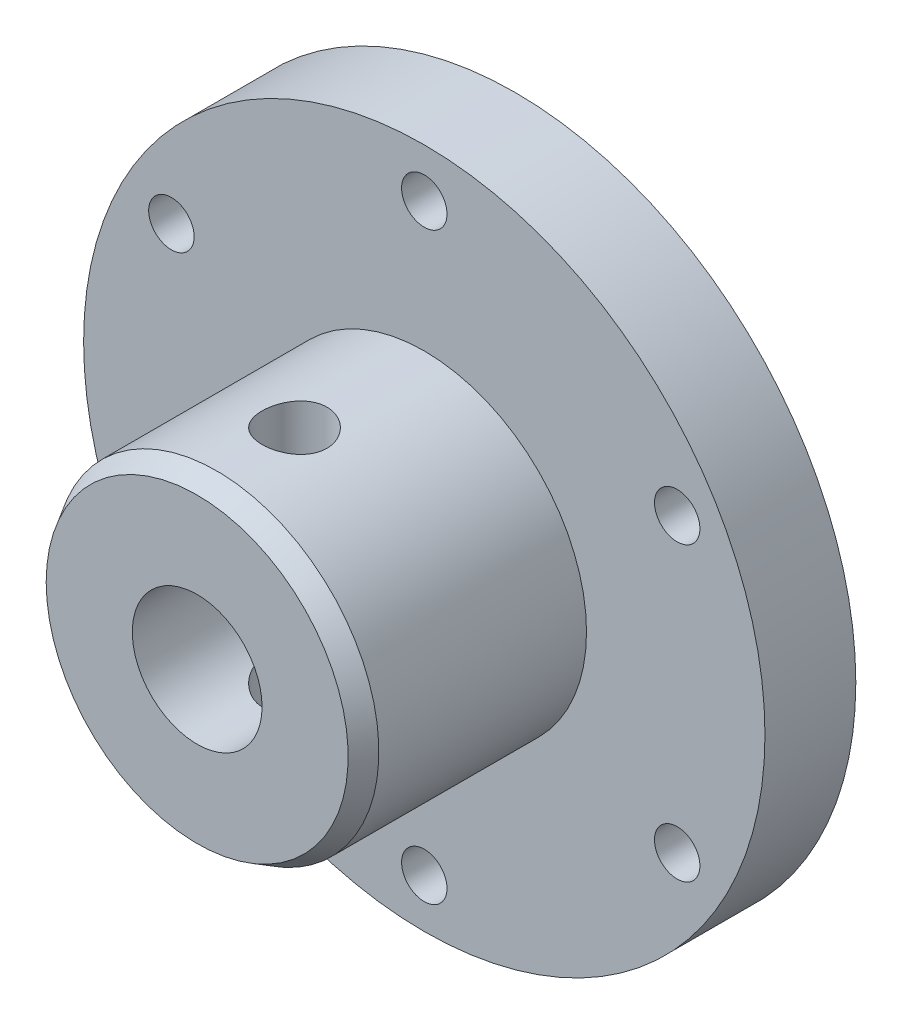
SolidWorks part; units mm, degrees
ref_plane "Front Plane" through (0, 0, 0) normal (0, 0, 1) x (1, 0, 0)
ref_plane "Top Plane" through (0, 0, 0) normal (0, 1, 0) x (1, 0, 0)
ref_plane "Right Plane" through (0, 0, 0) normal (1, 0, 0) x (0, 0, -1)
other "Configuration Table"
sketch "Sketch1" plane through (0, 0, 0) normal (0, 0, 1) x (1, 0, 0)
  circle A0 centre (0, 0) radius 52.5
  circle A1 centre (0, 0) radius 45 construction
  circle A2 centre (0, 45) radius 3.5
  circle A3 centre (38.9711, 22.5) radius 3.5
  circle A4 centre (38.9711, -22.5) radius 3.5
  circle A5 centre (0, -45) radius 3.5
  circle A6 centre (-38.9711, -22.5) radius 3.5
  circle A7 centre (-38.9711, 22.5) radius 3.5
  point P19 (0, 0)
  dimension "D1" = 105
  dimension "D2" = 90
  dimension "D3" = 7
  dimension "D4" = 6
extrude "Boss-Extrude1" add sketch "Sketch1" along normal blind 14
sketch "Sketch2" plane through (0, 0, 14) normal (0, 0, 1) x (1, 0, 0)
  circle A0 centre (0, 0) radius 25
  circle A1 centre (0, 0) radius 10
  dimension "D1" = 50
  dimension "D2" = 20
extrude "Boss-Extrude2" add sketch "Sketch2" along normal blind 35
sketch "Sketch3" plane through (0, 0, 0) normal (0, 1, 0) x (1, 0, 0)
  line L0 (-25, -14) -> (25, -14) construction
  circle A0 centre (0, -34) radius 5
  dimension "D1" = 10
  dimension "D2" = 20
extrude "Cut-Extrude1" cut sketch "Sketch3" against normal through all both and the other way through all
chamfer "Chamfer1" distance 3 angle 30 1 edges at (25, 0, 49)
